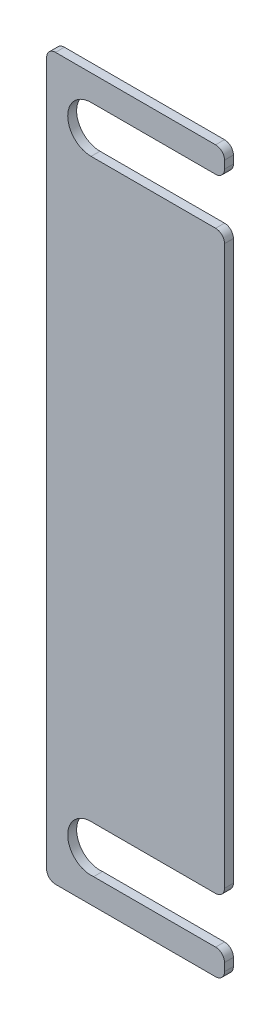
SolidWorks part; units mm, degrees
ref_plane "前视基准面" through (0, 0, 0) normal (0, 0, 1) x (1, 0, 0)
ref_plane "上视基准面" through (0, 0, 0) normal (0, 1, 0) x (1, 0, 0)
ref_plane "右视基准面" through (0, 0, 0) normal (1, 0, 0) x (0, 0, -1)
sketch "草图1" plane through (0, 0, 0) normal (0, 0, 1) x (1, 0, 0)
  line L1 (20, -81) -> (-20, -81)
  line L2 (20, -81) -> (20, 81)
  line L3 (20, 81) -> (-20, 81)
  line L4 (-20, -81) -> (-20, 81)
  line L5 (20, -81) -> (-20, 81) construction
  line L6 (20, 81) -> (-20, -81) construction
  point P0 (0, 0)
  dimension "D1" = 40
  dimension "D2" = 162
extrude "凸台-拉伸1" add sketch "草图1" along normal blind 2
sketch "草图2" plane through (0, 0, 2) normal (0, 0, 1) x (1, 0, 0)
  line L0 (-20, 81) -> (-20, -81) construction
  line L2 (-10, -70) -> (-10, 70) construction
  circle A2 centre (-10, 70) radius 5.25
  circle A3 centre (-10, -70) radius 5.25
  point P0 (-10, 0)
  dimension "D3" = 10.5
  dimension "D1" = 140
  dimension "D2" = 10
extrude "切除-拉伸1" cut sketch "草图2" against normal blind 3
sketch "草图4" plane through (0, 0, 2) normal (0, 0, 1) x (1, 0, 0)
  line L0 (20, -81) -> (20, 81) construction
  line L17 (-10, 64.75) -> (20, 64.75)
  line L18 (-10, 64.75) -> (-10, 75.25)
  line L19 (-10, 75.25) -> (20, 75.25)
  line L20 (20, 64.75) -> (20, 75.25)
  line L22 (-9.4344, -64.7806) -> (20, -64.7806)
  line L23 (-9.4344, -64.7806) -> (-9.4344, -75.2194)
  line L24 (-9.4344, -75.2194) -> (20, -75.2194)
  line L25 (20, -64.7806) -> (20, -75.2194)
  circle A0 centre (-10, 70) radius 5.25 construction
  circle A4 centre (-10, 70) radius 5.25 construction
  circle A5 centre (-10, -70) radius 5.25 construction
extrude "切除-拉伸4" cut sketch "草图4" against normal blind 10
fillet "圆角2" radius 2 8 edges at (-20, -81, 1) (-20, 81, 1) (20, -81, 1) (20, 81, 1) (20, -75.2194, 1) (20, -64.7806, 1) (20, 64.75, 1) (20, 75.25, 1)
